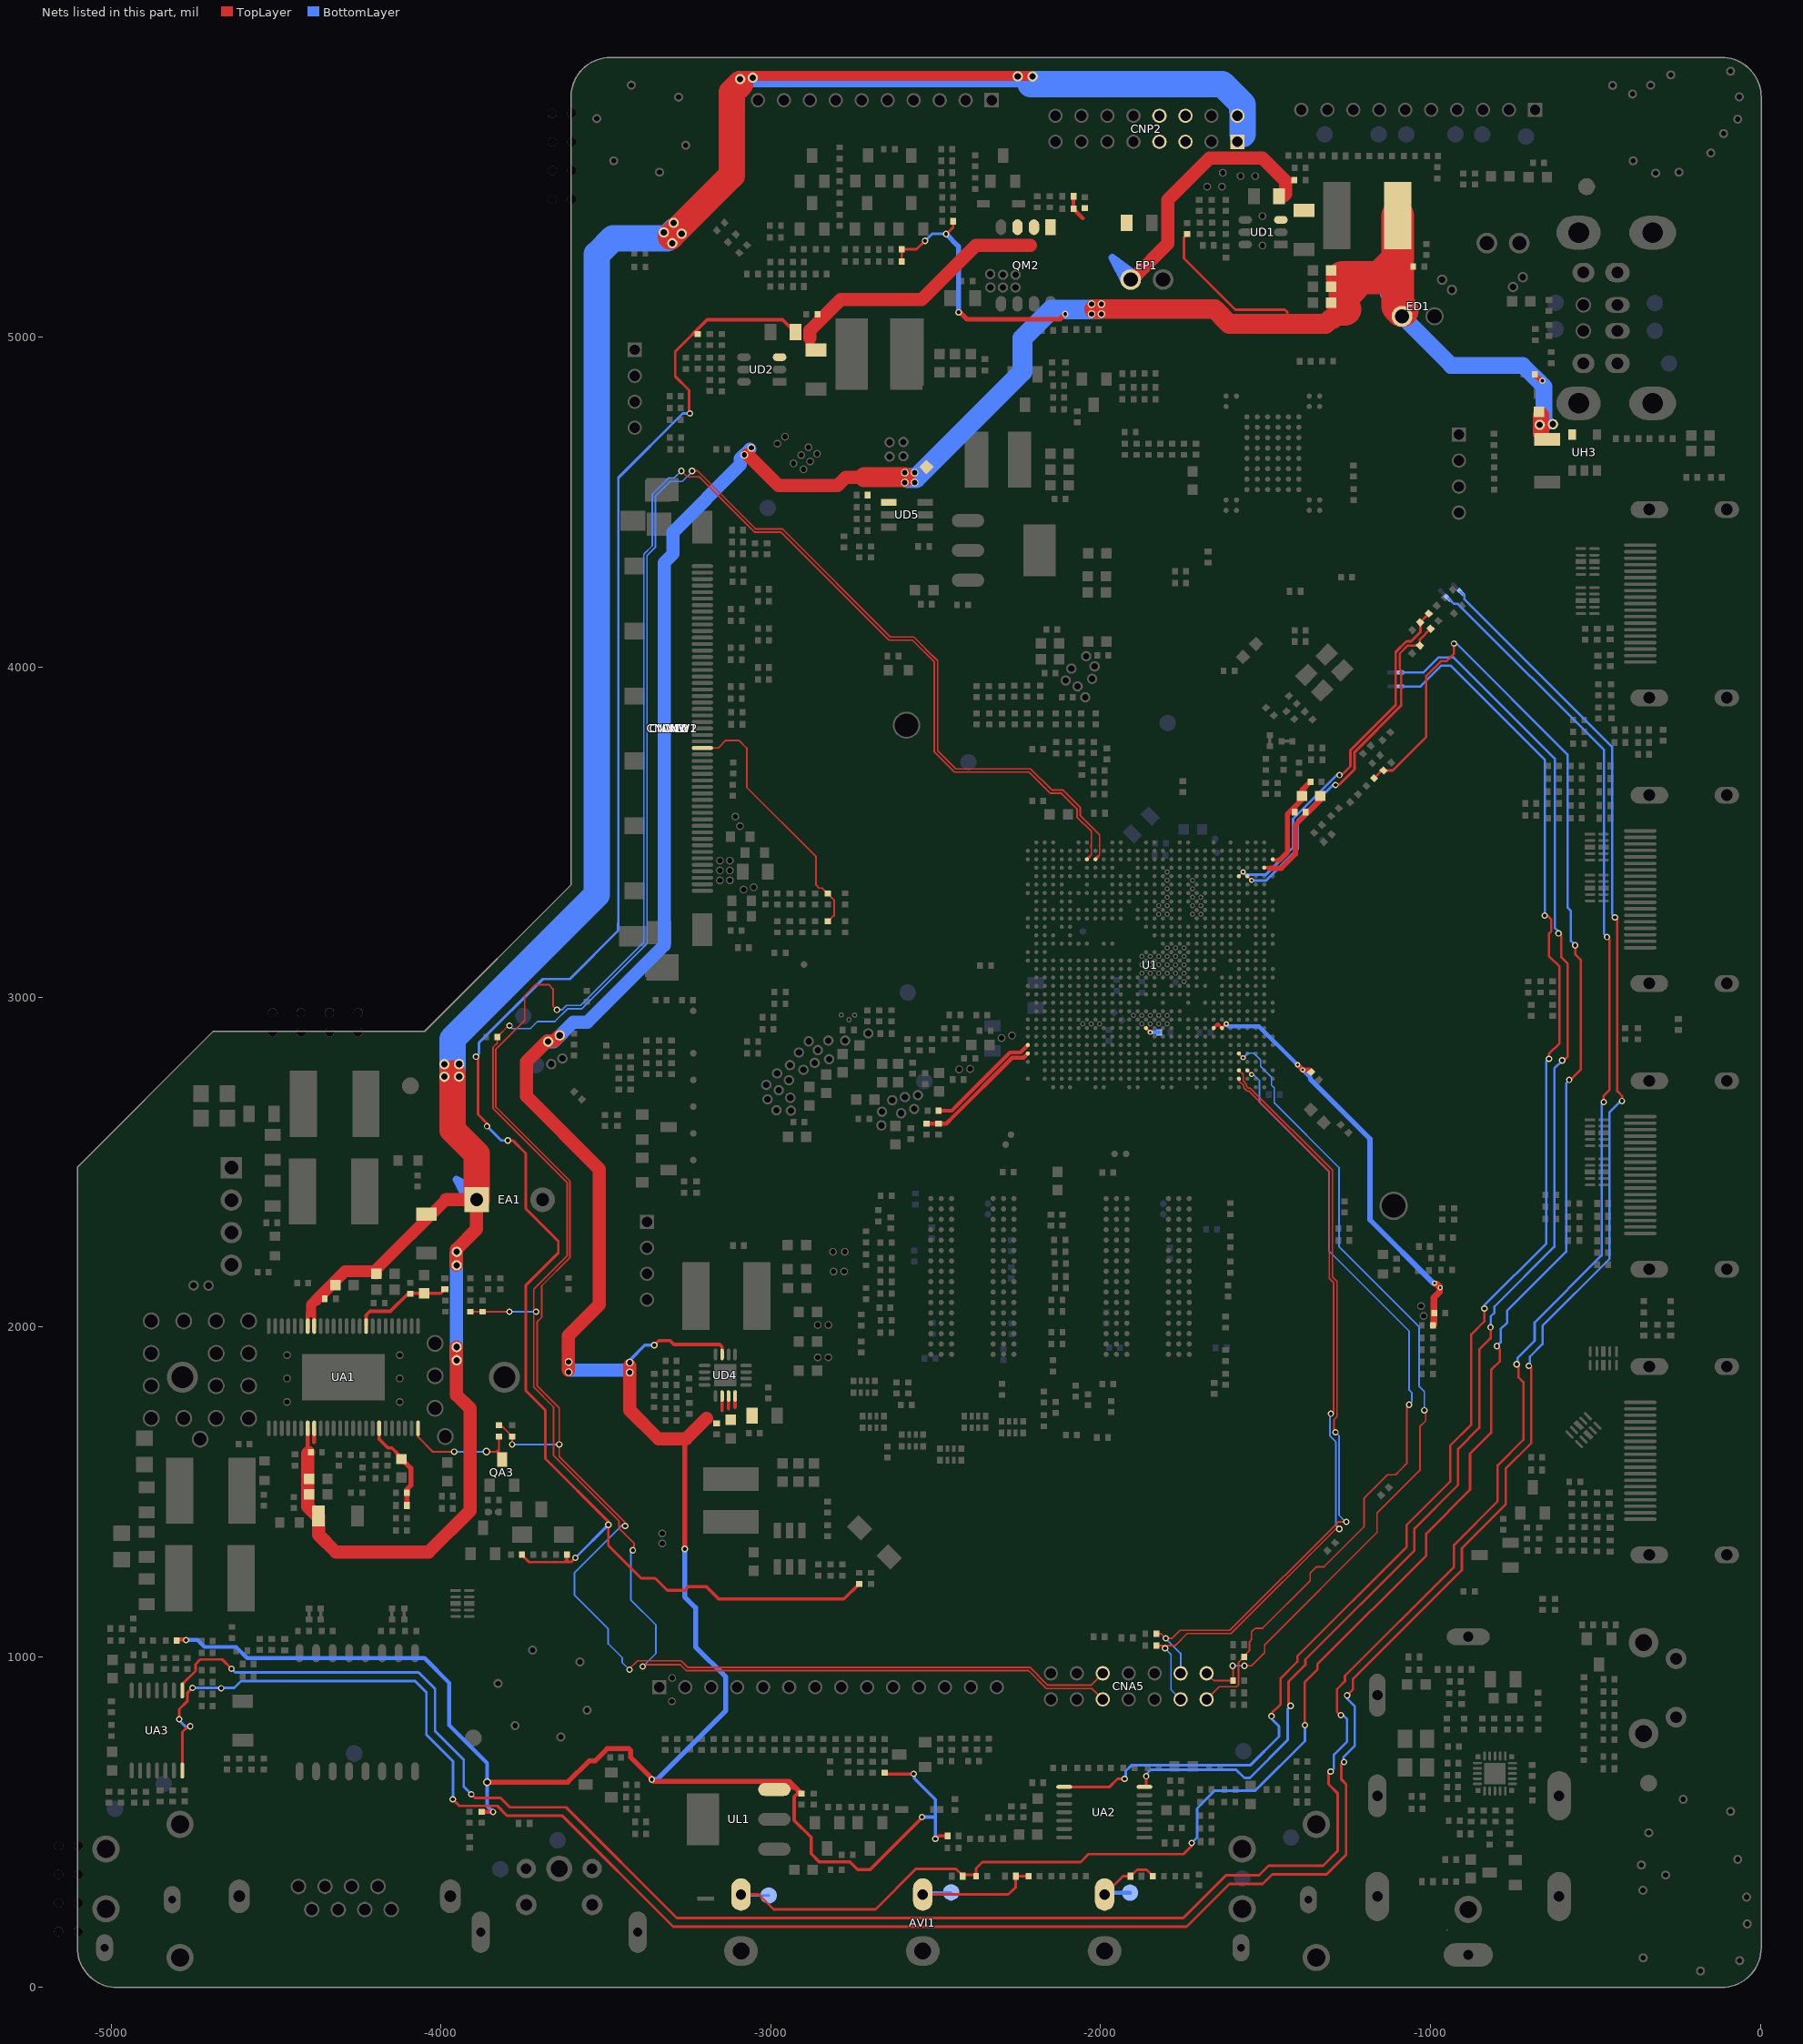
[diagram p0: the nets of this part, all layers, seen from the top]
# Altium PCB MISC86290.PcbDoc (part 10 of 31)
Units mil, origin at the board's own origin, x right, y up, seen from the top; angles counter-clockwise.
Board outline 5104.71 x 5851.49 mil, 2 copper layers (TopLayer, BottomLayer), stack 61.855 mil thick; 1026 components, 667 nets, 4280 pads, 2294 vias.

## Via types
v1: diameter 19.68, hole 11.81, TopLayer to BottomLayer, tented both sides, 1189 vias
v2: diameter 19.68/19.68 (per signal layer), hole 11.81, TopLayer to BottomLayer, tented both sides, 366 vias
v3: diameter 15.75, hole 7.87, TopLayer to BottomLayer, tented both sides, 348 vias
v4: diameter 23.62, hole 15.75, TopLayer to BottomLayer, tented both sides, 309 vias
v5: diameter 15.75/15.75 (per signal layer), hole 7.87, TopLayer to BottomLayer, tented both sides, 59 vias
v6: diameter 24/24 (per signal layer), hole 16, TopLayer to BottomLayer, tented both sides, 23 vias

## Nets (pads, with @x,y where several pads share a name; then routed paths per layer and width w, separated by ;. In a path a pad name is that pad's centre, name@x,y a point inside that pad or via, vN(x,y) a via of type N, cw(c..) or ccw(c..) an arc to the next point about the centre after c; other vN are vias at no path point) (continued)
5V_M: 5V_M.1 CD7.2 CD8.2 CD9.2 CD10.2 CD32.2 CD33.1 CD43.2 CD51.2 CL1.1 CU3.2 CU4.2 ED1.1 FU1.1 LD1.2 LD4.2 pad.VIA5@-629,4737 pad.VIA5@-669,4735 pad.VIA5@-1997.75,5070.84 pad.VIA5@-1997.75,5100.84 pad.VIA5@-2027.75,5070.84 pad.VIA5@-2027.75,5100.84 pad.VIA5@-2564,4560 pad.VIA5@-2564,4590 pad.VIA5@-2594,4560 pad.VIA5@-2594,4590 pad.VIA5@-3059.03,4665.21 pad.VIA5@-3080.25,4644 pad.VIA5@-3428,1862 pad.VIA5@-3428,1892 pad.VIA5@-3613,1863 pad.VIA5@-3613,1894 pad.VIA5@-3640,2884 pad.VIA5@-3675,2865 RD5.1 RD52.2 RG1.2 RG12.2 RG37.2 RK10.2 RO3.1 RO19.2 RO41.2 UD4.3 UD4.10 UD4.11 UD4.12 UD5.4 UH3.5 UL1.3 | length 13839.4
  TopLayer w8: RG12.2@-2603.27,5230.5 RG37.2@-2603.27,5267 -2558.5,5267 v1(-2532.5,5293) ; v1(-2468.6,5313.66) -2467.34,5313.66 -2447.52,5333.48 RG1.2@-2447.52,5352 ; RD5.1@-1737.47,5313.27 -1747.25,5303.49 -1747.25,5239.38 -1591.87,5084 -1441.5,5084 -1434,5076.5 -1434,5041
  TopLayer w10: v1@-3357,1945 v1@-3355.25,1946.75 ; v1(-3353.5,1945) -3339.66,1958.84 -3305.84,1958.84 -3294,1947 -3154.98,1947 -3147.85,1939.87 UD4.3@-3147.85,1916.68 ; -3147.85,1747.09 UD4.10@-3147.85,1790.7 ; -3128.17,1752.08 UD4.11@-3128.17,1790.7 ; -3108.48,1755.77 UD4.12@-3108.48,1790.7 ; CL1.1@-2916.56,588.68 -2929.37,575.88 -2929.37,504.37 -2878,453 -2878,402.95 -2853.37,378.31 -2760.31,378.31 -2737,355 -2699,355 -2542,512 v1(-2542,514.5) ; RK10.2@-2650.32,644.59 -2568.03,644.59 v1(-2567.03,645.59) ; v1(-2501,448) -2492,457 RO19.2@-2464.46,457
  TopLayer w12: RO41.2@-4800.78,1053 -4775,1053 v1(-4773,1051) ; RO3.1@-3876.25,530 v1(-3842.25,530)
  TopLayer w15: v4(-3860,620) -3615.43,620 -3550.93,684.5 -3533.17,684.5 -3496.17,721.5 -3430.55,721.5 -3424.55,715.5 -3424.55,695.35 -3361,631.81 v1(-3361,628) -3356,623 -2944.52,623 CL1.1@-2907.25,585.73 ; v1(-3261,1327) -3261,1652.48 ; UL1.3@-3015.97,586.55 UL1.3@-2985.98,586.55 ; UL1.3@-2989.25,598 -2982.25,605 -2927.52,605 -2911.2,588.68 CL1.1@-2916.56,588.68 ; v1(-2431,5076) -2425.71,5076 -2404.71,5055 -2123.45,5055 v1(-2107.56,5070.88) ; CU4.2@-684.27,4888 -665.27,4869 v1(-661,4869)
  TopLayer w40: pad.VIA5@-3642.5,2881 -3656.5,2867 -3677.17,2867 -3740.5,2803.67 -3740.5,2699.72 -3519.75,2478.97 -3519.75,2068.06 -3613.5,1974.31 pad.VIA5@-3613.5,1869.5 ; pad.VIA5@-3428,1883 pad.VIA5@-3428,1862 -3428,1748 -3341.5,1661.5 -3270.02,1661.5 ; -3256.89,1661.5 -3195.39,1723 ; pad.VIA5@-3070.76,4645.24 -2976.68,4551.16 -2797.84,4551.16 -2772.65,4576.35 -2717.25,4576.35
  TopLayer w50: FU1.1@-665.5,4709.46 CU3.2@-665.5,4764
  TopLayer w60: -2717.25,4576.35 -2594,4576.35 ; -2020.25,5085.66 -1655.16,5085.66 -1610.5,5041 -1434,5041 -1318.71,5041 -1304.37,5055.34 -1295.16,5055.34 -1265.25,5085.25 -1259.23,5091.27
  TopLayer w100: -1267.4,5181 -1210.32,5181 ; -1265.25,5085.25 -1259.23,5085.25 ; -1259.23,5132.1 -1210.32,5181 ; -1099.73,5215 -1099.73,5094.8 ED1.1@-1086.43,5081.5 ; LD4.2@-1099.73,5369 -1099.73,5236.5 -1155.23,5181 -1210.32,5181
  BottomLayer w8: v1(-2532.5,5293) -2511.84,5313.66 v1(-2468.6,5313.66) v1@-2465.76,5316.5
  BottomLayer w10: pad.VIA5@-3426.75,1890.75 -3426.75,1900.25 -3382,1945 v1@-3357,1945 ; v1(-2567.03,645.59) -2564.25,642.82 -2564.25,630.75 -2501,567.5 v1(-2501,448) ; v1(-2542,514.5) -2501.5,514.5
  BottomLayer w12: v1(-4773,1051) -4737.99,1051 -4716.99,1030 -4621.37,1030 -4587.37,996 -4049.91,996 -3975,921.09 -3975,792.8 -3860,677.8 v4(-3860,620) -3860,547.75 v1(-3842.25,530)
  BottomLayer w15: v1(-3361,628) -3345.5,628 -3136.56,836.94 -3136.56,889.64 ; v1(-3261,1327) -3261,1182 -3228.25,1149.25 -3228.25,1030.25 -3136.56,938.56 -3136.56,926.36 ; -3136.49,889.71 -3136.49,926.29 ; v1(-2468.6,5313.66) -2431,5276.05 v1(-2431,5076)
  BottomLayer w40: pad.VIA5@-3675,2865 -3658.51,2865 -3598.99,2924.51 -3555.83,2924.51 -3323.61,3156.74 -3323.61,4317.11 -3297.25,4343.48 -3297.25,4409 -3092.25,4614 -3092.25,4631.95 pad.VIA5@-3063.1,4661.1 ; pad.VIA5@-3605,1869.5 pad.VIA5@-3430.5,1869.5
  BottomLayer w50: ED1.1@-1086.43,5064 5V_M.1@-937.46,4915 -720.65,4915 -656.16,4850.5 pad.VIA5@-656.16,4737
  BottomLayer w60: -2585.25,4574 -2559.25,4574 -2237.25,4896 -2237.25,4997 -2149.75,5084.5 -2027.75,5084.5 -2007.5,5084.5
12V: CD1.2 CD2.2 CD3.1 CD11.1 CD12.2 CD13.2 CM15.2 CNP2.5 CNP2.6 CNP2.7 CNP2.8 CP1.2 CP2.2 EP1.1 QM2.1 QM2.2 QM2.3 R120.2 RA22.1 RA24.2 RD11.1 RM13.1 UD1.3 UD2.3 | length 7498.5
  TopLayer w8: v1(-3894,2819.5) -3887.8,2813.3 -3887.8,2644.37 -3860.5,2617.07 v1(-3860.5,2608.5) ; v1(-3797.5,2565.5) -3782.21,2565.5 -3742.5,2525.79 -3742.5,2408.15 -3743.37,2407.28 -3743.37,2358.87 -3644.15,2259.65 -3644.15,2224.85 -3743.3,2125.7 -3743.3,1807.96 -3683.34,1748 -3683.34,1600.57 -3492.66,1409.88 v1(-3492.66,1400.11) -3492.66,1337.53 -3393.13,1238 -3350.78,1238 -3315.78,1203 -3313.36,1203 ; RA24.2@-3753.25,1307.25 -3733.16,1287.16 -3625,1287.16 ; RA22.1@-3618.27,1310 -3618.27,1293.89 ; v1(-3592.74,1300.03) -3605.61,1287.16 -3611.54,1287.16 ; v1(-3245.5,4769.5) -3247.5,4771.5 -3247.5,4839.49 -3290,4881.99 -3290,4957.3 -3237.57,5009.73 ; -3625,1287.16 -3611.54,1287.16 ; -3625,1287.16 -3618.27,1293.89 ; -3618.27,1293.89 -3611.54,1287.16
  TopLayer w10: -3313.36,1202 -3260.92,1202 -3250.58,1212.34 -3195.34,1212.34 -3158.18,1175.18 -2778.24,1175.18 R120.2@-2732.16,1221.27 ; -3237.57,5009.73 -3193.7,5053.61 -2964.61,5053.61 -2935,5024 CD11.1@-2925.25,5024
  TopLayer w12: CM15.2@-2082.52,5390 RM13.1@-2082.52,5428 ; CM15.2@-2080.52,5387 -2054.52,5361
  TopLayer w40: -2882,4997.5 -2882,5020.6 -2788.1,5114.5 -2543,5114.5 -2378.5,5279 -2213.25,5279 ; EP1.1@-1903,5183 -1898,5183 -1796.25,5284.75 -1796.25,5416.4 -1669.3,5543.35 -1509.35,5543.35 -1439,5473 -1439,5435.23 CD3.1@-1444.39,5429.83
  BottomLayer w8: v1(-3894,2819.5) -3884.5,2829 -3884.5,2861.65 -3691.15,3055 -3609.19,3055 -3462.61,3201.58 -3462.61,3223.44 -3462.11,3223.94 -3462.11,4574.43 -3267.04,4769.5 v1(-3245.5,4769.5) ; v1(-3860.5,2608.5) -3817.5,2565.5 v1(-3797.5,2565.5) ; v1(-3592.74,1300.03) v1(-3492.66,1400.11)
AGND-HPL: RO18.JP_1K UA2.14 | length 4503.2
  TopLayer w7: v1@-1424.16,849.84 -1430.5,856.18 -1430.5,925.17 -1379.49,976.18 -1379.49,992.17 -1049.09,1322.57 -1049.09,1388.88 -916.28,1521.68 -916.28,1630.36 -852.34,1694.3 -852.34,1931.57 -817.66,1966.25 -817.66,1998.66 v1(-818,1999) ; v1(-612,3193) -608.34,3193 -604.34,3189 -604.34,3121.55 -585,3102.21 -585,2819 -596,2808 v1(-601,2808)
  TopLayer w8: UA2.14@-1867.44,605.77 -1862,611.22 v1(-1862,638)
  BottomLayer w7: RO18.JP_1K@-1093.24,3984 -1022,3984 -976.66,4029.34 -929.4,4029.34 -623.34,3723.28 -623.34,3210.34 -612,3199 v1(-612,3193) ; v1(-818,1999) -818,2031.76 -805.94,2043.82 -805.94,2062.09 -625,2243.03 -625,2784 v1(-601,2808)
  BottomLayer w8: v1(-1862,638) -1862,644.01 -1848.01,658 -1589.5,658 -1564.5,633 -1548.08,633 -1433.16,747.92 -1433.16,842.31 v1(-1424.16,851.31)
AGND-HPR: RO17.JP_1K UA2.1 | length 4673.9
  TopLayer w7: v1@-1484,820 -1484,827.29 -1454.5,856.79 -1454.5,935.11 -1403.66,985.95 -1403.66,1001.94 -1073.09,1332.51 -1073.09,1398.82 -940.28,1531.63 -940.28,1640.31 -876.34,1704.24 -876.34,1977.34 -837,2016.69 v1(-837,2056) ; v1(-654,3247) -646,3247 -634,3235 -634,3199.68 -641.34,3192.34 -641.34,3124.61 -609,3092.27 -609,2859.94 -641.34,2827.6 -641.34,2813.34 v1(-641,2813)
  TopLayer w8: UA2.1@-2110.55,605.77 -1973,605.77 -1948.77,630 v1(-1927.5,630) ; v1@-1484,820 v1(-1482,820)
  BottomLayer w7: RO17.JP_1K@-1093.24,3942 -1029.94,3942 ; -1028.94,3943 -966.6,4005.34 -939.34,4005.34 -654,3720 v1(-654,3247) ; v1(-837,2056) -837,2064.97 -649,2252.97 -649,2805 v1(-641,2813)
  BottomLayer w8: v1(-1927.5,630) -1924.5,633 -1924.5,653.5 -1907,671 -1546.85,671 -1459.16,758.69 -1459.16,789.16 -1482,812 v1(-1482,820)
AGND-LL: RO36.JP_1K UA3.14 | length 8795.9
  TopLayer w7: v1(-1253,883) -1235.49,900.51 -1235.49,932.52 -905.09,1262.92 -905.09,1329.23 -772.28,1462.04 -772.28,1570.72 -694.88,1648.12 -694.88,1876.88 v1@-702,1884 ; v1(-441,3242) -434,3235 -434,2715 -419,2700 -419,2686 v1(-420,2685)
  TopLayer w8: v1(-4793.34,811.04) -4793.34,841.1 -4769.24,865.21 -4769.24,890.2 v1(-4753.22,906.22) ; UA3.14@-4784.14,655.21 -4784.14,772.1 ; v1@-4768.25,788 -4784.14,772.1 ; v1(-4760.12,789.48) -4766.76,789.48 -4784.14,772.1 ; v1(-3964,568) -3944,548 -3935,548 -3829.25,548 -3799.25,518 -3631.61,518 -3295.93,182.32 -3289.18,182.32 ; -3287.93,182.32 -1739.15,182.32 -1609.46,312 -1509,312 -1480,341 -1315.25,341 -1256,400.25 -1256,614 -1270,628 -1270,676 -1265,681 v1(-1262,681)
  BottomLayer w7: v1@-1264,681 -1264,696 -1229.66,730.34 -1229.66,849.66 -1253,873 v1(-1253,883) ; RO36.JP_1K@-908.09,4228.09 -898,4218 -898,4206.91 -450,3758.91 -450,3251 v1(-441,3242) ; v1@-702,1884 -699,1884 -699,1909.71 -660.54,1948.16 -660.54,2003.84 -457.5,2206.88 -457.5,2651.45 -423.95,2685 v1(-420,2685)
  BottomLayer w8: v1(-4793.34,811.04) -4793.34,807.34 -4775.48,789.48 v1(-4760.12,789.48) ; v1(-4753.22,906.22) -4626.78,906.22 -4606,927 -4078.49,927 -4044,892.51 -4044,764.22 -3964,684.22 v1(-3964,568) ; v1@-1264,681 v1(-1262,681)
  other v1: -4666.25,905 -702,1882
AGND-LR: RO35.JP_1K UA3.1 | length 8521.2
  TopLayer w7: v1(-1272,823) -1274,823 -1283.66,832.66 -1283.66,902.31 -1259.49,926.48 -1259.49,942.47 -929.09,1272.86 -929.09,1339.17 -796.28,1471.98 -796.28,1580.66 -718.88,1658.06 -718.88,1832.94 -733,1847.06 -733,1881 v1(-739,1887) ; v1(-475,2682) -475,2701 -458,2718 -458,3175 v1(-465,3182) v1@-462,3185
  TopLayer w8: UA3.1@-4784.14,898.32 -4784.14,917.44 -4744.25,957.34 -4744.25,977.66 -4729.91,992 -4663,992 v1(-4635,964) ; v1(-3908,583) -3897,572 -3819.31,572 -3791.31,544 -3620.85,544 -3285.16,208.32 -1749.91,208.32 -1620.23,338 -1519.77,338 -1490.77,367 -1326.01,367 -1282,411.01 -1282,587 -1309,614 -1309,650 -1307,652 v1(-1303,652)
  BottomLayer w7: v1(-1303,652) -1292.66,662.34 -1292.66,703.34 -1253.66,742.34 -1253.66,811.66 -1265,823 v1(-1272,823) ; RO35.JP_1K@-945.62,4208.63 -929.07,4192.07 -917.1,4192.07 -474,3748.97 -474,3191 v1(-465,3182) ; v1(-739,1887) -736,1887 -736,1906.65 -684.54,1958.1 -684.54,2013.78 -481.5,2216.82 -481.5,2675.5 v1(-475,2682)
  BottomLayer w8: v1(-4635,964) -4624,953 -4067.72,953 -4018,903.28 -4018,774.99 -3931,687.99 -3931,607 -3908,584 v1(-3908,583)
AGP: CNW1.29 CNW2.29 CNW3.29 CNW12.29 RW409.1 RW416.2 | length 803.6
  TopLayer w5: CNW3.29@-3207.67,3755.47 -3159.21,3755.47 -3136.33,3778.34 -3096.53,3778.34 -3072.75,3754.56 -3072.75,3635.49 -2863,3425.75 -2863,3340 -2853.62,3330.62 -2844.13,3330.62 RW416.2@-2827.5,3314 -2808.25,3294.75 -2808.25,3247.52 -2826.77,3229 RW409.1@-2827.5,3228.27
AMP_AVDD1: CA15.2 CA16.2 LA12.2 UA1.18 | length 266.5
  TopLayer w10: UA1.18@-4187.48,1692.73 -4187.48,1660.34 -4160.6,1633.46 -4148.97,1633.46 CA16.2@-4130.11,1614.6
  TopLayer w15: CA16.2@-4119.75,1599.62 -4091.5,1571.37 -4091.5,1520.15 -4104,1507.65 -4104,1459.74 LA12.2@-4103.26,1459
AMP_DVDD1: CA9.2 CA10.2 LA10.2 UA1.33 | length 304.6
  TopLayer w10: UA1.33@-4226.85,2002.77 -4226.85,2036.15 -4215.5,2047.5 -4153.5,2047.5 -4098.81,2102.19 CA10.2@-4051,2102.19 -4000.07,2102.19 LA10.2@-3988,2114.26
AMP_MUTEN: CNA5.9 RA9.2 RA20.2 U1.AH23 | length 8138.5
  TopLayer w3.94: -2034.83,3424.73 -2028.86,3430.71 -2028.86,3452.36
  TopLayer w5: RA9.2@-3824,1701.73 -3817.46,1701.73 RA20.2@-3784,1668.27 v1(-3784,1644) ; v1(-3648.5,2961.5) -3660.32,2973.32 -3660.32,3024.87 -3673.47,3038.03 -3712.97,3038.03 -3746.4,3004.6 -3746.4,2929.44 -3833.6,2842.24 -3833.6,2666.82 -3608.85,2442.06 -3608.85,2210.66 -3694.66,2124.85 -3694.66,2029.13 -3708.8,2014.99 -3708.8,1822.25 -3641.5,1754.95 v1(-3641.5,1644) -3641.5,1607.52 -3441.5,1407.52 v1(-3441.5,1397) ; v1@-3428.5,964.16 -3404.5,988.16 -3271.98,988.16 -3252.14,968.31 -2214.7,968.31 -2160.39,914 -2029.74,914 CNA5.9@-1993.74,950 ; v1(-3271,4595) -3253.36,4577.36 -3217.03,4577.36 -3049.01,4409.34 -2968.73,4409.34 -2641.39,4082 -2570.85,4082 -2504.5,4015.65 -2504.5,3743.1 -2443.51,3682.11 -2216.59,3682.11 -2152.48,3618 -2118.89,3618 -2071.9,3571.01 -2071.9,3546.24 -2028.15,3502.5 -2028.15,3462.8 ; -2028.86,3452.36 -2028.86,3462.09
  TopLayer w10: U1.AH23@-2041.65,3417.91 -2034.83,3424.73
  BottomLayer w5: v1(-3784,1644) v1(-3641.5,1644) ; v1(-3648.5,2961.5) -3633.42,2961.5 -3619.91,2975.01 -3576.75,2975.01 -3385.11,3166.65 -3385.11,4342.65 -3359.5,4368.26 -3359.5,4524.5 -3309.5,4574.5 -3292.27,4574.5 -3271,4595.77 v1(-3271,4595) ; v1@-3448.36,1401.5 -3595.5,1254.36 -3595.5,1187.5 -3493,1085 -3493,1039.73 -3450.5,997.23 -3450.5,983 v1(-3428.5,961)
AMP_PDN1: QA3.C RA9.1 UA1.24 | length 404.6
  TopLayer w6: UA1.24@-4069.37,1692.73 -4069.37,1666.05 -4025.32,1622 v1(-3960,1622) ; v4(-3862,1622) -3831,1622 ; RA9.1@-3824,1668.27 -3824,1629 ; QA3.C@-3814.5,1598.5 QA3.C@-3814.5,1598.03 ; -3831,1622 QA3.C@-3824,1615 ; -3831,1622 -3824,1629 ; QA3.C@-3824,1615 -3824,1604.53 -3814.5,1595.03 QA3.C@-3814.5,1598.03 ; QA3.C@-3824,1615 -3814.5,1605.5 QA3.C@-3814.5,1598.03 ; QA3.C@-3824,1615 -3824,1629
  BottomLayer w6: v1(-3960,1622) v4(-3862,1622)
AMP_RSTN: CNA5.10 RA11.2 RA21.1 RA34.2 U1.AH22 | length 7908.8
  TopLayer w3.94: -2008.98,3425 -2003.27,3430.71 -2003.27,3450.11
  TopLayer w5: RA21.1@-3911,2046.27 RA11.2@-3874,2046.27 v1(-3792.73,2046.27) ; v1(-3792,2913.5) -3795.27,2913.5 RA34.2@-3829.27,2879.5 -3829.27,2860.71 -3842.5,2847.48 -3842.5,2663.13 -3617.75,2438.38 -3617.75,2215.2 -3718.8,2114.14 -3718.8,1818.1 -3658.84,1758.15 -3658.84,1610.72 -3460,1411.87 -3460,1389.5 -3414.5,1344 -3414.5,1327 v1(-3418.5,1323) ; v1@-3383,976 -3273.96,976 -3256.28,958.31 -2218.84,958.31 -2164.53,904 -2026.48,904 CNA5.10@-1993.74,871.26 ; v2@-3239,4596 -3222.94,4596 -3046.28,4419.34 -2964.59,4419.34 -2637.24,4092 -2566.71,4092 -2499.25,4024.54 ; -2509.91,4035.2 -2494.5,4019.79 -2494.5,3747.24 -2439.37,3692.11 -2213,3692.11 ; -2212.45,3692.11 -2148.34,3628 -2114.75,3628 -2061.9,3575.15 -2061.9,3550.39 -2003.27,3491.75 -2003.27,3450.11
  TopLayer w10: U1.AH22@-2016.06,3417.91 -2008.98,3425
  BottomLayer w5: v1(-3792.73,2046.27) v1@-3711.73,2046.27 ; v1(-3792,2913.5) -3783,2904.5 -3729,2904.5 -3707.5,2926 -3654.78,2926 -3615.77,2965.01 -3572.61,2965.01 -3375.61,3162.01 -3375.61,4338.71 -3349.75,4364.58 -3349.75,4518.75 -3305,4563.5 -3268.5,4563.5 v2@-3238,4594 ; v1(-3418.5,1323) -3424,1317.5 -3424,1171.93 -3348.25,1096.18 -3348.25,1010.75 v1(-3388.5,970.5)
  other v1: -3711.5,2046.5
  other v2: -3239,4595
AMP_VCC: CA1.2 CA2.2 CA4.2 CA6.2 CA8.2 CA12.2 CA30.2 CA31.2 CNP2.1 CNP2.2 EA1.1 pad.VIA5@-2206.5,5791 pad.VIA5@-2251.5,5791.5 pad.VIA5@-3054.69,5787.5 pad.VIA5@-3093.07,5782.96 pad.VIA5@-3270.5,5314.5 pad.VIA5@-3294.5,5347.5 pad.VIA5@-3298.5,5285.5 pad.VIA5@-3324.5,5318.5 pad.VIA5@-3945,2759 pad.VIA5@-3945,2797 pad.VIA5@-3952,2228 pad.VIA5@-3952.5,1899 pad.VIA5@-3952.5,1939.22 pad.VIA5@-3952.5,2187 pad.VIA5@-3989.5,2758.79 pad.VIA5@-3989.5,2796.79 UA1.7 UA1.8 UA1.41 UA1.42 | length 9208.7
  TopLayer w11.8: -4403.9,1633.87 UA1.7@-4403.9,1692.73 ; UA1.42@-4403.9,1994.89 -4403.9,1998.83 -4403.9,2045 ; -4384.45,1650.87 UA1.8@-4384.45,1692.73 ; UA1.41@-4384.45,1994.89 -4384.45,1998.83 -4384.45,2045
  TopLayer w30: -4394,2045 -4394,2068.45 -4362.89,2099.56 ; -3118.5,5767.53 -3093.07,5792.96 pad.VIA5@-2208.65,5792.96
  TopLayer w35: -4378.26,2081.76 -4356.63,2103.39 -4356.36,2103.39 -4291,2168.75 CA12.2@-4204.06,2168.75 ; CA12.2@-4196.31,2161 -4202.91,2167.59 -3984.5,2386
  TopLayer w40: CA2.2@-4401.33,1619.39 -4404.39,1616.34 -4404.39,1455.52 CA31.2@-4371.44,1422.57 ; CA31.2@-4371.44,1427.47 CA31.2@-4371.44,1422.57 ; -3984.5,2386 EA1.1@-3892,2386 -3892,2296 -3952.5,2235.5 pad.VIA5@-3952.5,2187 ; pad.VIA5@-3952.5,1939.22 pad.VIA5@-3952.5,1899 -3952.5,1793.51 -3912,1753.01 -3912,1443 -4036.84,1318.16 -4319.16,1318.16 -4371.44,1370.44 CA31.2@-4371.44,1422.57
  TopLayer w80: -3965.33,2769 -3965.33,2598.33 -3892,2525 EA1.1@-3892,2386 ; -3303.21,5306.34 -3118.5,5491.05 -3118.5,5742.53 pad.VIA5@-3093.07,5767.96
  BottomLayer w40: pad.VIA5@-3952.5,1904 pad.VIA5@-3952.5,1939.22 pad.VIA5@-3952.5,2187 pad.VIA5@-3952.5,2225
  BottomLayer w50: pad.VIA5@-3093.07,5782.96 -2227.82,5782.96 -2212.82,5767.96
  BottomLayer w80: -3965.33,2769 -3965.33,2872.75 -3527.11,3310.97 -3527.11,5251.69 -3478.46,5300.34 -3314.16,5300.34 -3291.5,5323 ; -2212.82,5767.96 -1631.25,5767.96 -1569.25,5705.96 CNP2.2@-1569.25,5685 ; CNP2.2@-1570.88,5686.63 CNP2.2@-1569.25,5685 ; -1569.25,5616 CNP2.2@-1569.25,5685
AU_DAC_L: CO51.2 RO51.1 U1.AF5 | length 1108.5
  TopLayer w4.92: U1.AF5@-1581.02,3366.73 v3(-1568.23,3379.53)
  TopLayer w8: v1(-1276,3673) -1269.35,3673 -1243,3699.35 -1243,3748.56 -1105.84,3885.72 -1105.84,4046.34 -1073.18,4079 -1059,4079 -1031,4107 -1031,4135.71 CO51.2@-1031.74,4136.44 RO51.1@-1005.19,4162.98
  BottomLayer w8: v3(-1568.23,3379.53) -1559.51,3370.81 -1500.19,3370.81 -1417,3454 -1417,3540.73 -1280.37,3677.37 v1(-1276,3673)
AU_DAC_R: CO52.2 RO52.1 U1.AF4 | length 1070.6
  TopLayer w3.94: U1.AF4@-1555.43,3366.73 v3(-1542.64,3353.94)
  TopLayer w7: -1089,3884.18 -1089,3991 -1093.34,3995.34 -1093.34,4041.16 -1068.67,4065.83 CO52.2@-1032.17,4065.83 ; CO52.2@-1032.84,4066.5 CO52.2@-1032.17,4065.83 ; RO52.1@-999.83,4117.17 -1032.17,4084.83 CO52.2@-1032.17,4065.83
  TopLayer w8: v1(-1288,3643) -1287,3644 -1277,3644 -1230,3691 -1230,3743.18 -1089,3884.18
  BottomLayer w8: v3(-1542.64,3353.94) -1498.06,3353.94 -1403,3449 -1403,3536.35 -1294.35,3645 -1290,3645 v1(-1288,3643)
AUBCK_OUT: CNA5.2 RA3.1 U1.C4 | length 2439
  TopLayer w5: CNA5.2@-1678.78,871.26 -1640.71,909.33 -1588.1,909.33 -1582,915.42 -1582,983.27 RA3.1@-1565.27,1000 -1565.27,1003.73 -1548.91,1020.09 -1548.91,1046.09 -1542.69,1052.31 -1542.69,1075.74 -1531.93,1086.5 -1509.5,1086.5 -1364.84,1231.16 -1364.84,1253.59 -1345.43,1273 -1323,1273 -1202.01,1393.99 -1202.01,1480.06 -1130.07,1552 -1106.14,1552 -1090.32,1567.82 -1072.22,1585.92 -1072.22,1757.13 v1(-1064.88,1764.47) ; U1.C4@-1555.43,2778.15 v3(-1542.64,2765.35)
  BottomLayer w5: v3@-1537.05,2765.35 -1527.05,2755.35 ; -1526.94,2755.25 -1518.63,2746.94 -1518.63,2681.74 -1307.67,2470.78 -1307.67,2229.84 -1064.88,1987.05 -1064.88,1808.88 -1056.66,1800.66 -1056.66,1773.93 ; v1@-1065.5,1765.09 -1056.96,1773.63
AUMCK_OUT: CNA5.1 RA4.1 U1.E5 | length 2540.1
  TopLayer w3.94: U1.E5@-1581.02,2829.33 v3(-1568.23,2816.54)
  TopLayer w5: CNA5.1@-1678.78,950 -1656.78,928 RA4.1@-1598.73,928 -1598.73,971.73 v1(-1600,973) ; v1(-1564,973) -1542.47,973 -1503,1012.47 -1503,1036.54 -1162.09,1377.45 -1162.09,1435.68 -1032.3,1565.47 -1032.3,1697.55 -1014.52,1715.34 -1014.52,1742.87 v1(-1019,1747.35)
  BottomLayer w3.94: v3(-1568.23,2816.54) -1554.45,2830.31 -1536.34,2830.31 -1515.13,2809.11 -1515.13,2790.19
  BottomLayer w5: v1(-1600,973) v1(-1564,973) ; -1515.13,2790.19 -1482,2757.06 -1482,2733 -1474,2725 -1474,2679.74 -1277.67,2483.41 -1277.67,2244.05 -1034.96,2001.34 -1034.96,1820.37 -1019,1804.41 v1(-1019,1747.35)
AUSD_OUT: CNA5.3 RA1.1 U1.C5 | length 2367.9
  TopLayer w3.94: U1.C5@-1581.02,2778.15 -1568.23,2765.35 -1568.23,2745.53 -1558.39,2735.69 -1558.39,2729.92 -1552.48,2724.02 -1546.57,2724.02 -1297.72,2475.17 -1297.72,2471.25
  TopLayer w5: RA1.1@-1831.27,1070 -1817,1070 v1(-1803,1056) -1784,1056 -1759.39,1080.61 -1608.53,1080.61 -1280.02,1409.12 v1(-1255.5,1409.12) ; -1297.2,2471.25 -1297.2,2151.2 -1283.72,2137.72 -1283.72,1728.94 -1292.34,1720.33 -1292.34,1685.34 v1(-1288,1681)
  BottomLayer w5: v1(-1803,1056) -1757.52,1010.52 CNA5.3@-1757.52,950 ; v1(-1288,1681) -1277.5,1670.5 -1277.5,1429.5 -1257.12,1409.12 v1(-1255.5,1409.12)
AUVAG: CO4.2 CO5.2 U1.AG2 | length 322.9
  TopLayer w10: U1.AG2@-1504.25,3392.32 -1490,3392.32
  TopLayer w16: -1488.32,3390.65 -1452.46,3390.65 -1410,3433.11 -1410,3521.65 -1333.19,3598.46 CO5.2@-1333.19,3614
AUVRM: CO4.1 CO5.1 LO1.1 U1.AH1 | length 289
  TopLayer w10: U1.AH1@-1478.66,3417.91 -1475.71,3414.96 -1463.9,3414.96
  TopLayer w16: -1463.9,3414.96 -1457.85,3414.96 -1433.82,3438.99 -1433.82,3554.59 CO5.1@-1388.81,3599.6 ; CO5.1@-1389.81,3610 -1389.81,3627.19 LO1.1@-1364,3653
AUWS_OUT: CNA5.4 RA2.1 U1.B5 | length 2387.6
  TopLayer w3.94: U1.B5@-1581.02,2752.56 -1581.02,2746.65 -1566.26,2731.89 -1566.26,2725.98 -1556.42,2716.14 -1551.13,2716.14 -1306.72,2471.73
  TopLayer w5: RA2.1@-1829.86,1035.41 RA2.1@-1831.27,1034 -1774.5,1034 -1737.89,1070.61 -1604.39,1070.61 -1287.01,1387.98 v1(-1276.63,1387.98) ; -1307.2,2471.25 -1307.2,2147.06 -1293.72,2133.58 -1293.72,1743.28 -1300,1737 v1(-1302,1737)
  BottomLayer w5: v1(-1805,1026) -1786.67,1007.67 -1786.67,900.41 CNA5.4@-1757.52,871.26 ; v1@-1298,1733 v1(-1302,1737) -1305.34,1733.66 -1305.34,1670.34 -1287.5,1652.5 -1287.5,1398.85 v1(-1276.63,1387.98)
AV_IN: AV_IN.1 AVI1.1 CI1.2 DI1.K RI1.1 RI2.2 | length 6485.2
  TopLayer w7: v1@-1381.16,794.84 -1381.16,923.6 -1343.49,961.27 -1343.49,977.26 -1013.09,1307.66 -1013.09,1373.97 -880.28,1506.77 -880.28,1615.45 -816.34,1679.39 -816.34,1869.54 -790,1895.88 -790,1933 v1(-799,1942) ; RI1.1@-1171.17,3663.83 -1147.83,3687.17 RI2.2@-1142.83,3687.17 -1114.83,3687.17 -1013,3789 -1013,3974.5 -969.15,4018.34 -951.66,4018.34 -929,4041 v1(-929,4072) ; v1@-576,2749 -544,2781 -544,3112.12 -560.88,3129 v1@-560.88,3156
  TopLayer w8: AVI1.1@-3091.8,279.53 -3091.27,279 AVI1.1@-3090.55,279 ; AVI1.1@-3090.55,279.53 -3036.49,279.53 -2991.28,234.32 -2682.75,234.32 -2559.4,357.67 -2439.56,357.67 -2420.73,338.84 -2377.73,338.84 -2377.73,358.78 -2358.67,377.84 -2060.93,377.84 -2036.77,402 -1749,402 -1724,427 v1(-1724,436)
  BottomLayer w7: v1@-924.49,4075.34 -585,3735.85 -585,3272.22 -574.34,3261.56 -574.34,3169.46 v1(-562,3157.12) ; v1(-799,1942) -787.34,1953.66 -787.34,1993.57 -768.54,2012.37 -768.54,2048.57 -589,2228.12 -589,2738 v1@-580,2747
  BottomLayer w8: AVI1.1@-3091.8,279.53 -3088.77,276.5 AV_IN.1@-3006.75,276.5 ; v1(-1724,436) -1708.04,451.96 -1708.04,540.58 -1677.32,571.3 -1654.62,594 -1531.92,594 -1381,744.92 v1(-1381,793)
  other v1: -580,2749
AV_L: AV_L.1 AVI1.3 DI2.K RI3.1 | length 457.3
  TopLayer w8: AVI1.3@-2546.75,285.65 AVI1.3@-2540.62,279.53 ; AVI1.3@-2539.37,279.53 -2279.47,279.53 -2257.27,301.73 DI2.K@-2257.27,335 RI3.1@-2221.73,335
  BottomLayer w8: AVI1.3@-2539.37,279.53 -2532.9,286 AV_L.1@-2453.5,286
AV_R: AV_R.1 AVI1.5 DI3.K RI6.1 | length 265.3
  TopLayer w8: AVI1.5@-1988.19,279.53 -1932.72,335 DI3.K@-1909.73,335 -1908.68,335 -1889.68,354 -1860.73,354 RI6.1@-1841.73,335
  BottomLayer w8: AVI1.5@-1988.66,280 AVI1.5@-1988.19,279.53
  BottomLayer w12: AVI1.5@-1988.19,279.53 -1982.72,285 AV_R.1@-1911,285
AVDD_DDR_VBN_B_SM: C49.2 U1.F30 | length 352.6
  TopLayer w11.81: C49.2@-2491,2656 -2451.2,2656 -2437.78,2669.43 -2274.92,2832.28 -2243.43,2832.28 U1.F30@-2220.79,2854.92
AVDD_DDR_VBP_B_DM: C46.1 U1.H16 | length 45.3
  TopLayer w7.87: U1.H16@-1862.52,2906.1 v3(-1849.72,2893.31)
  BottomLayer w11.81: v3(-1849.72,2893.31) C46.1@-1822.48,2893.31
AVDD_DDR_VBP_B_SM: C47.2 C48.2 U1.E30 | length 395.9
  TopLayer w11.81: C48.2@-2528.5,2616.5 C47.2@-2491.5,2616.5 -2468.26,2616.5 -2447.01,2637.74 -2268.22,2816.54 -2233.58,2816.54 U1.E30@-2220.79,2829.33
AVDD_EAR33/AU33: C30.2 C111.2 pad.VIA5@-970.44,2119 pad.VIA5@-988,2133 pad.VIA5@-1387.45,2779.45 pad.VIA5@-1403.01,2795.01 R3.2 U1.H7 U1.H8 | length 1359.5
  TopLayer w9.84: U1.H8@-1657.8,2906.1 -1645,2918.9 U1.H7@-1632.2,2906.1 v3(-1619.41,2918.9)
  TopLayer w15.75: pad.VIA5@-1403.01,2795.01 pad.VIA5@-1388.83,2780.83 ; pad.VIA5@-1387.45,2779.45 -1368.45,2779.45 C111.2@-1361.98,2772.98
  TopLayer w20: R3.2@-993,2004.84 -990.05,2007.8 -990.05,2089.07 -972.74,2106.38 -972.74,2121.63 -981.28,2130.17 pad.VIA5@-985.16,2130.17
  BottomLayer w10: v3@-1619.41,2918.68 v3(-1619.41,2918.9)
  BottomLayer w13: v3@-1619.41,2918.68 -1612.46,2911.73 -1520.28,2911.73 pad.VIA5@-1407.03,2798.48 ; pad.VIA5@-1403.01,2795.01 -1364,2756
  BottomLayer w15.75: -1364,2750.98 -1183.5,2570.48 -1183.5,2324.59 -989.95,2131.05 -979.99,2131.05 pad.VIA5@-970.44,2121.5